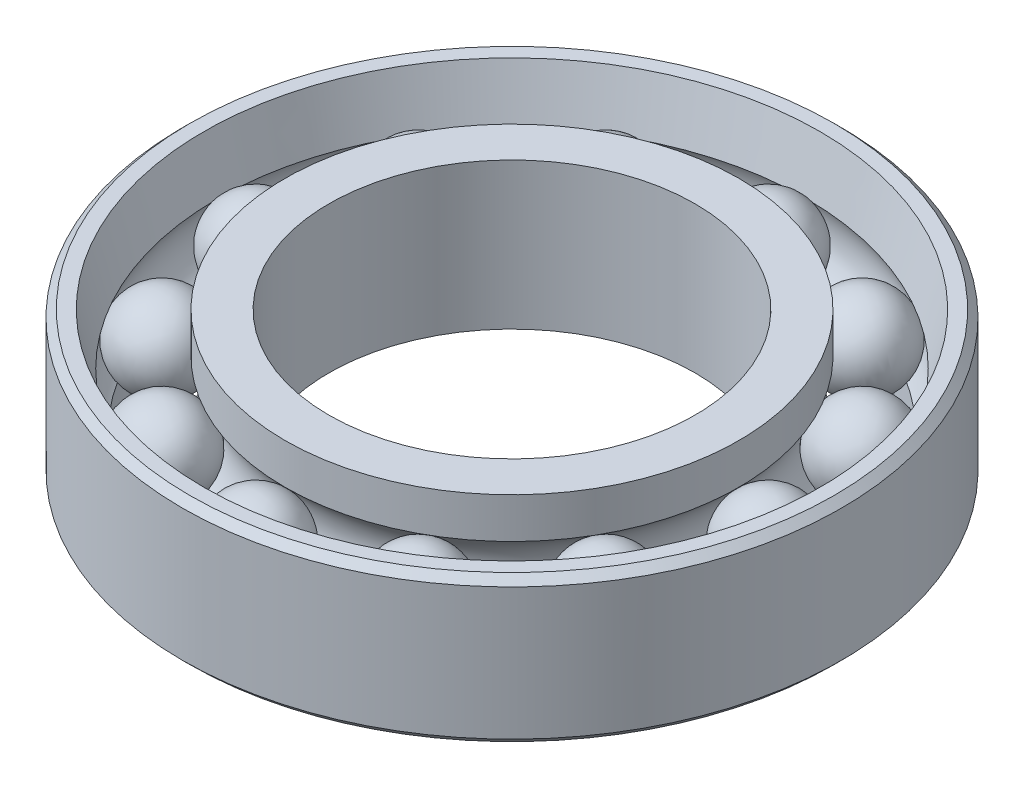
from build123d import *

# Parameters (mm, degrees)
CHAMFER1_SIZE = 1


with BuildPart() as part:
    # Sketch1 → Revolve1 (revolve)
    with BuildSketch(Plane.XY, mode=Mode.PRIVATE) as revolve1_sk:
        with BuildLine():
            Line((-25, 10), (-31, 10))
            Line((-31, 10), (-31, 4.472135955))
            ThreePointArc((-31, 4.472135955), (-29, 0), (-31, -4.472135955))
            Line((-31, -4.472135955), (-31, -10))
            Line((-31, -10), (-25, -10))
            Line((-25, -10), (-25, 10))
        make_face()
        with BuildLine():
            Line((-45, 10), (-45, -10))
            Line((-45, -10), (-39, -10))
            Line((-39, -10), (-39, -4.472135955))
            ThreePointArc((-39, -4.472135955), (-40.924568236, -0.948415111), (-40.196152423, 3))
            Line((-40.196152423, 3), (-42.07179677, 10))
            Line((-42.07179677, 10), (-45, 10))
        make_face()
    revolve(revolve1_sk.sketch.rotate(Axis((0, 0, 0), (0, -1, 0)), 270), axis=Axis((0, 0, 0), (0, -1, 0)))

    # Chamfer1
    chamfer1_edges = [part.edges().sort_by_distance(p)[0] for p in [
        (0, -10, -45),
        (0, 10, -45),
    ]]
    chamfer(chamfer1_edges, length=CHAMFER1_SIZE)


with BuildPart() as body_2:
    # Sketch2 → Revolve2 (revolve)
    with BuildSketch(Plane(origin=(0, 0, 0), x_dir=(1, 0, 0), z_dir=(0, 1, 0))):
        with BuildLine():
            Line((0, 29), (0, 41))
            ThreePointArc((0, 41), (6, 35), (0, 29))
        make_face()
    revolve(axis=Axis((0, 0, -29), (0, 0, -1)))


with BuildPart() as body_3:
    # Sketch3 → Revolve3 (revolve)
    with BuildSketch(Plane(origin=(0, 0, 0), x_dir=(1, 0, 0), z_dir=(0, 1, 0))):
        with BuildLine():
            Line((-14.5, 25.11473671), (-20.5, 35.507041555))
            ThreePointArc((-20.5, 35.507041555), (-12.303847577, 33.310889132), (-14.5, 25.11473671))
        make_face()
    revolve(axis=Axis((-14.5, 0, -25.11473671), (-0.5000000000000014, 0, -0.8660254037844379)))


with BuildPart() as body_4:
    # Sketch4 → Revolve4 (revolve)
    with BuildSketch(Plane(origin=(0, 0, 0), x_dir=(1, 0, 0), z_dir=(0, 1, 0))):
        with BuildLine():
            Line((-25.11473671, 14.5), (-35.507041555, 20.5))
            ThreePointArc((-35.507041555, 20.5), (-27.310889132, 22.696152423), (-25.11473671, 14.5))
        make_face()
    revolve(axis=Axis((-25.11473671, 0, -14.5), (-0.8660254037844399, 0, -0.49999999999999784)))


with BuildPart() as body_5:
    # Sketch6 → Revolve6 (revolve)
    with BuildSketch(Plane(origin=(0, 0, 0), x_dir=(1, 0, 0), z_dir=(0, 1, 0))):
        with BuildLine():
            Line((-35.507041555, -20.5), (-25.11473671, -14.5))
            ThreePointArc((-25.11473671, -14.5), (-33.310889132, -12.303847577), (-35.507041555, -20.5))
        make_face()
    revolve(axis=Axis((-35.507041555, 0, 20.5), (0.866025403784436, 0, -0.5000000000000047)))


with BuildPart() as body_6:
    # Sketch7 → Revolve7 (revolve)
    with BuildSketch(Plane(origin=(0, 0, 0), x_dir=(1, 0, 0), z_dir=(0, 1, 0))):
        with BuildLine():
            Line((-20.5, -35.507041555), (-14.5, -25.11473671))
            ThreePointArc((-14.5, -25.11473671), (-22.696152423, -27.310889132), (-20.5, -35.507041555))
        make_face()
    revolve(axis=Axis((-20.5, 0, 35.507041555), (0.4999999999999949, 0, -0.8660254037844416)))


with BuildPart() as body_7:
    # Sketch8 → Revolve8 (revolve)
    with BuildSketch(Plane(origin=(0, 0, 0), x_dir=(1, 0, 0), z_dir=(0, 1, 0))):
        with BuildLine():
            Line((0, -29), (0, -41))
            ThreePointArc((0, -41), (-6, -35), (0, -29))
        make_face()
    revolve(axis=Axis((0, 0, 29), (0, 0, 1)))


with BuildPart() as body_8:
    # Sketch9 → Revolve9 (revolve)
    with BuildSketch(Plane(origin=(0, 0, 0), x_dir=(1, 0, 0), z_dir=(0, 1, 0))):
        with BuildLine():
            Line((14.5, 25.11473671), (20.5, 35.507041555))
            ThreePointArc((20.5, 35.507041555), (12.303847577, 33.310889132), (14.5, 25.11473671))
        make_face()
    revolve(axis=Axis((14.5, 0, -25.11473671), (0.5000000000000011, 0, -0.866025403784438)))


with BuildPart() as body_9:
    # Sketch10 → Revolve10 (revolve)
    with BuildSketch(Plane(origin=(0, 0, 0), x_dir=(1, 0, 0), z_dir=(0, 1, 0))):
        with BuildLine():
            Line((25.11473671, 14.5), (35.507041555, 20.5))
            ThreePointArc((35.507041555, 20.5), (27.310889132, 22.696152423), (25.11473671, 14.5))
        make_face()
    revolve(axis=Axis((25.11473671, 0, -14.5), (0.8660254037844397, 0, -0.4999999999999981)))


with BuildPart() as body_10:
    # Sketch11 → Revolve11 (revolve)
    with BuildSketch(Plane(origin=(0, 0, 0), x_dir=(1, 0, 0), z_dir=(0, 1, 0))):
        with BuildLine():
            Line((29, 0), (41, 0))
            ThreePointArc((41, 0), (35, 6), (29, 0))
        make_face()
    revolve(axis=Axis((29, 0, 0), (1, 0, 0)))


with BuildPart() as body_11:
    # Sketch12 → Revolve12 (revolve)
    with BuildSketch(Plane(origin=(0, 0, 0), x_dir=(1, 0, 0), z_dir=(0, 1, 0))):
        with BuildLine():
            Line((25.11473671, -14.5), (35.507041555, -20.5))
            ThreePointArc((35.507041555, -20.5), (33.310889132, -12.303847577), (25.11473671, -14.5))
        make_face()
    revolve(axis=Axis((25.11473671, 0, 14.5), (0.8660254037844363, 0, 0.5000000000000043)))


with BuildPart() as body_12:
    # Sketch13 → Revolve13 (revolve)
    with BuildSketch(Plane(origin=(0, 0, 0), x_dir=(1, 0, 0), z_dir=(0, 1, 0))):
        with BuildLine():
            Line((14.5, -25.11473671), (20.5, -35.507041555))
            ThreePointArc((20.5, -35.507041555), (22.696152423, -27.310889132), (14.5, -25.11473671))
        make_face()
    revolve(axis=Axis((14.5, 0, 25.11473671), (0.49999999999999484, 0, 0.8660254037844417)))


with BuildPart() as body_13:
    # Sketch14 → Revolve14 (revolve)
    with BuildSketch(Plane(origin=(0, 0, 0), x_dir=(1, 0, 0), z_dir=(0, 1, 0))):
        with BuildLine():
            Line((-41, 0), (-29, 0))
            ThreePointArc((-29, 0), (-35, 6), (-41, 0))
        make_face()
    revolve(axis=Axis((-41, 0, 0), (1, 0, 0)))


solid = Compound([part.part, body_2.part, body_3.part, body_4.part, body_5.part, body_6.part, body_7.part, body_8.part, body_9.part, body_10.part, body_11.part, body_12.part, body_13.part])
